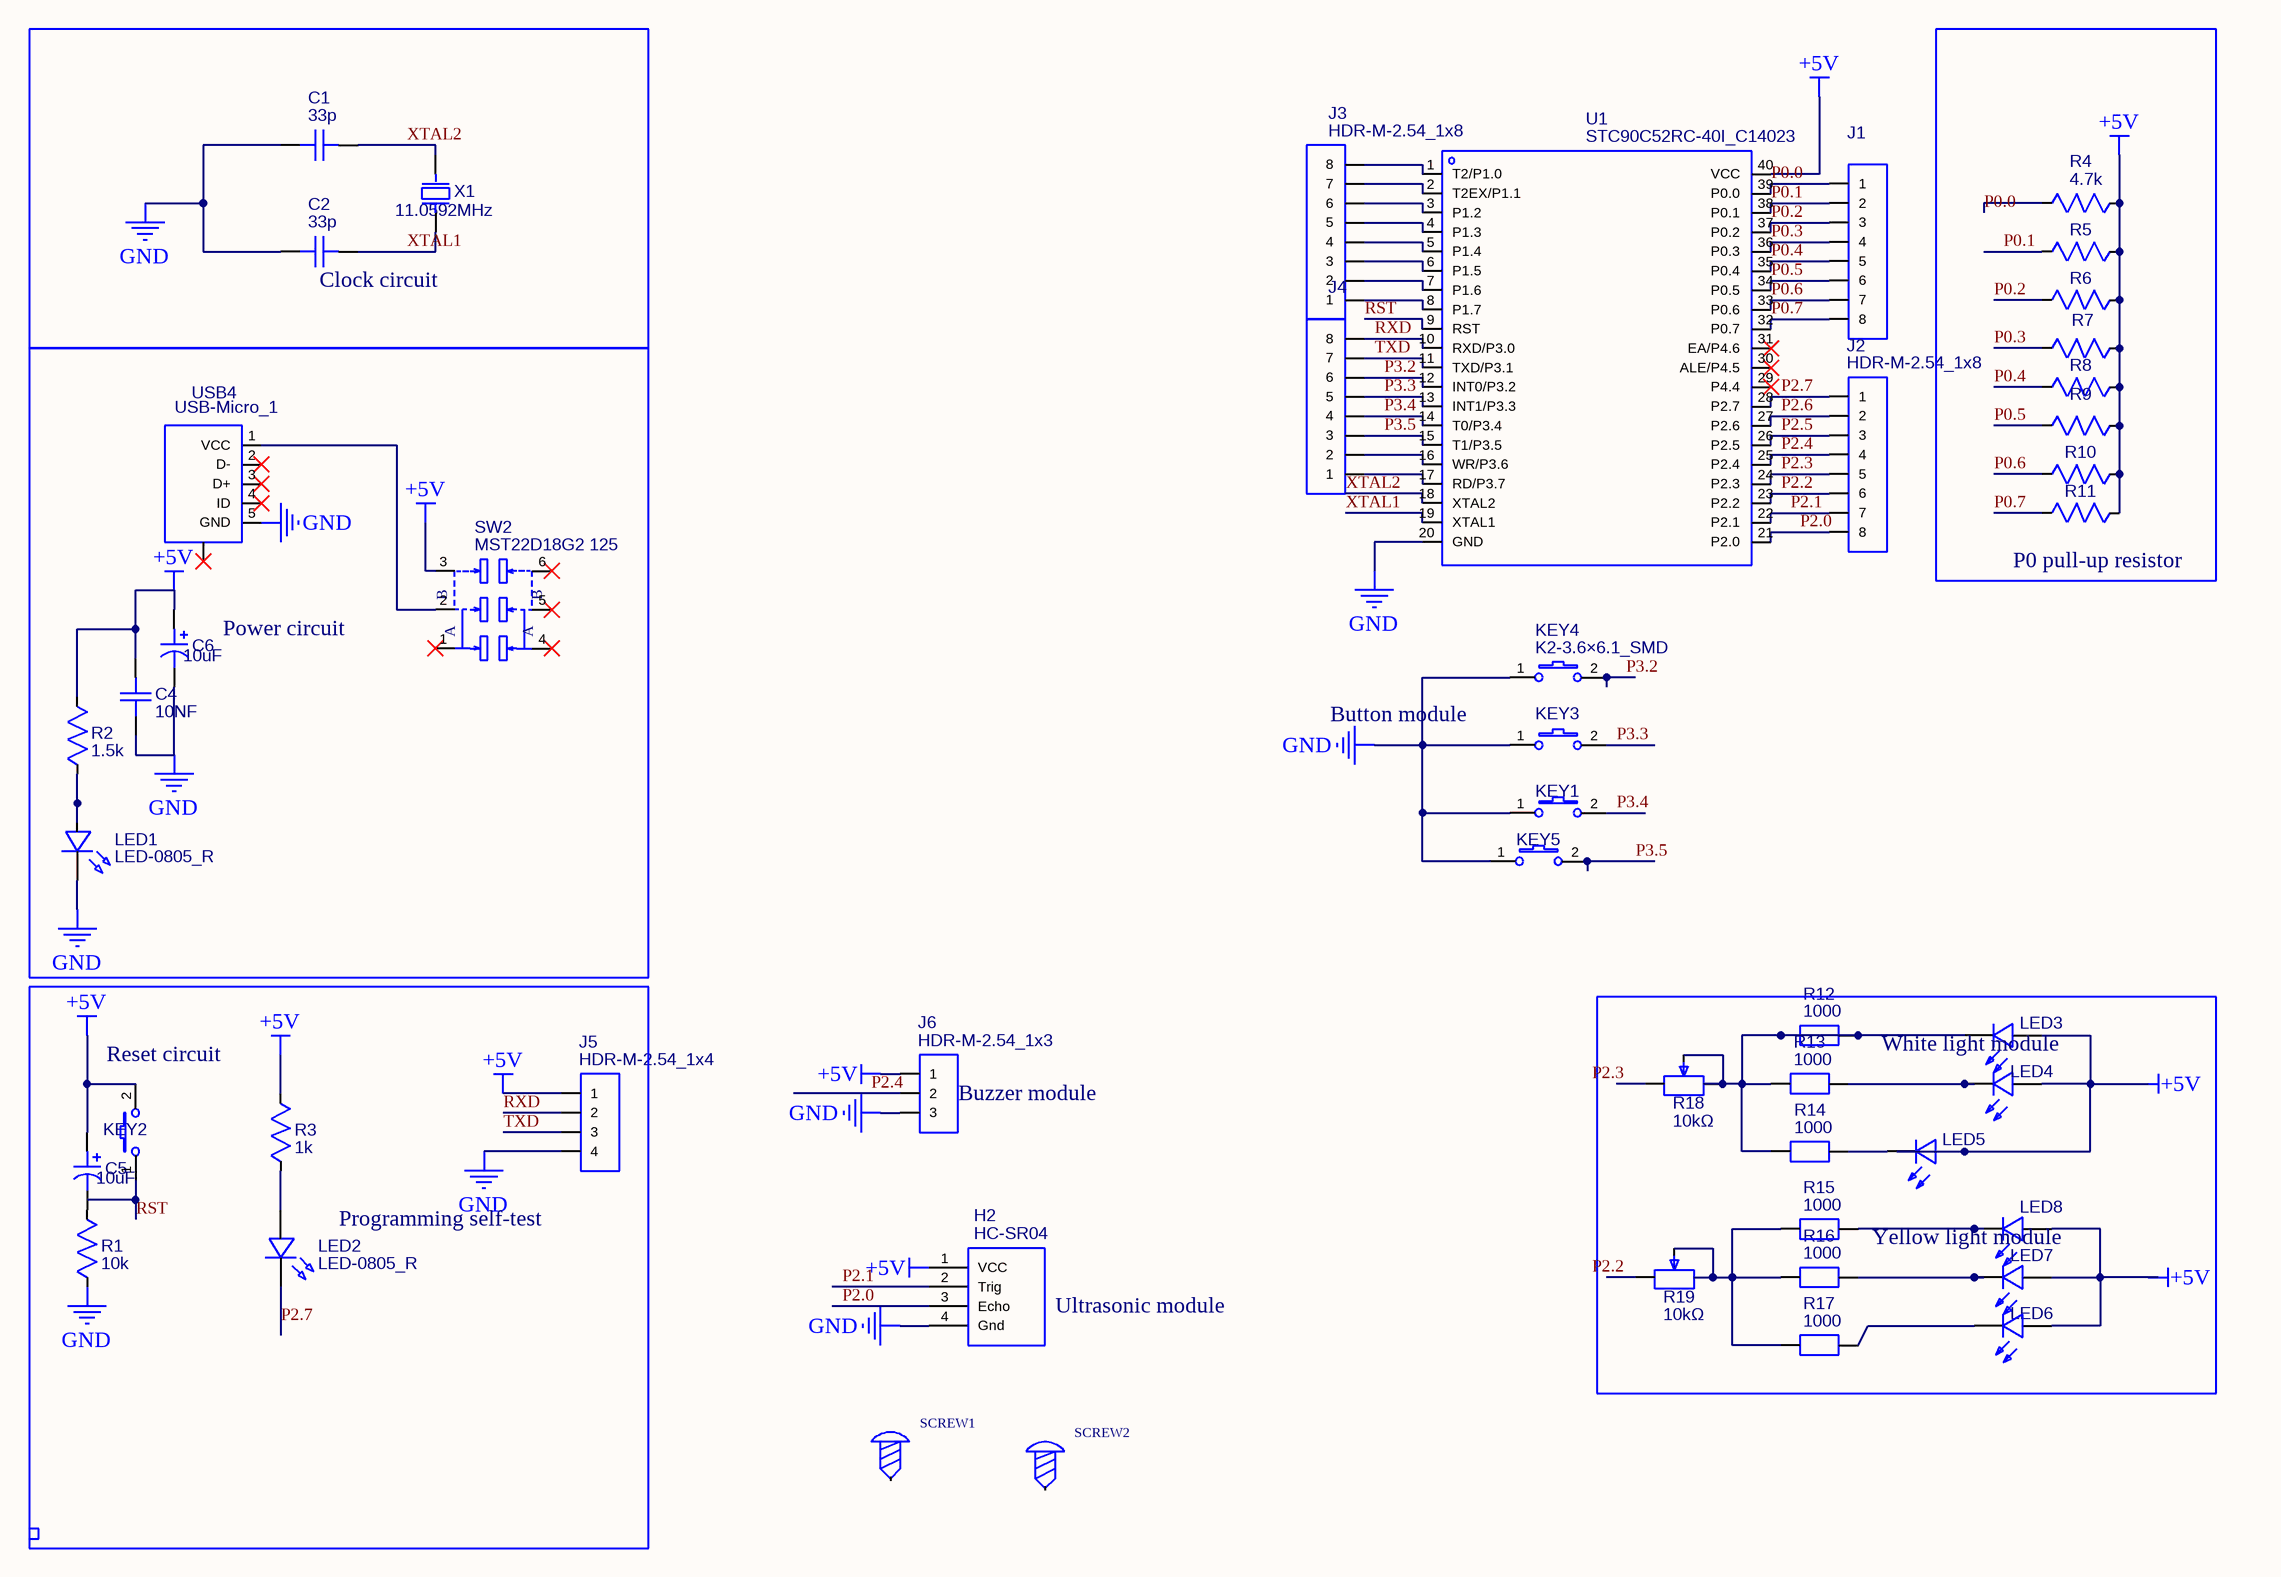
[diagram p0: MISC49914-3.schdoc]
# Altium project MISC49914-2.PrjPcb
1 sheet, 50 parts. Net scope: global (net labels, ports and power ports of the same name join across sheets).
Board file: MISC49914.pcbdoc

## Sheet MISC49914-3.schdoc
size 122 x 122 mm; Name: MISC49914; @Project Name: MISC49914; REV: 1.0; Date: 2023-03-04; Sheet: 1/1; Name: MISC49914; @Project Name: MISC49914; REV: 1.0; Date: 2023-03-04; Sheet: 1/1

### Parts
C1  33p  [C0805]
C2  33p  [C0805]
C4  10NF  [C0805]
C5  10uF  [CAP-TH_BD10.0-P5.00-D1.0-FD]
C6  10uF  [CAP-TH_BD10.0-P5.00-D1.0-FD]
H2  HC-SR04  [HC-SR04]
J1  HDR-M-2.54_1x8  [HDR-M-2.54_1X8]  (value not drawn)
J2  HDR-M-2.54_1x8  [HDR-M-2.54_1X8]
J3  HDR-M-2.54_1x8  [HDR-M-2.54_1X8]
J4  HDR-M-2.54_1x8  [HDR-M-2.54_1X8]  (value not drawn)
J5  HDR-M-2.54_1x4  [HDR-M-2.54_1X4]
J6  HDR-M-2.54_1x3  [HDR-M-2.54_1X3]
KEY1  K2-3.6×6.1_SMD  [KEY-SMD_2P-L6.2-W3.6-LS8.0]  (value not drawn)
KEY2  K2-3.6×6.1_SMD  [KEY-SMD_2P-L6.2-W3.6-LS8.0]  (value not drawn)
KEY3  K2-3.6×6.1_SMD  [KEY-SMD_2P-L6.2-W3.6-LS8.0]  (value not drawn)
KEY4  K2-3.6×6.1_SMD  [KEY-SMD_2P-L6.2-W3.6-LS8.0]
KEY5  K2-3.6×6.1_SMD  [KEY-SMD_2P-L6.2-W3.6-LS8.0]  (value not drawn)
LED1  LED-0805_R  [LED0805_RED]
LED2  LED-0805_R  [LED0805_RED]
LED3  204-10SDRD/S530-A3-L  [LED-TH_BD3.8-P2.54-FD]  (value not drawn)
LED4  204-10SDRD/S530-A3-L  [LED-TH_BD3.8-P2.54-FD]  (value not drawn)
LED5  204-10SDRD/S530-A3-L  [LED-TH_BD3.8-P2.54-FD]  (value not drawn)
LED6  204-10SDRD/S530-A3-L  [LED-TH_BD3.8-P2.54-FD]  (value not drawn)
LED7  204-10SDRD/S530-A3-L  [LED-TH_BD3.8-P2.54-FD]  (value not drawn)
LED8  204-10SDRD/S530-A3-L  [LED-TH_BD3.8-P2.54-FD]  (value not drawn)
R1  10k  [R0805]
R2  1.5k  [R0805]
R3  1k  [R0805]
R4  4.7k  [R0805]
R5  4.7k  [R0805]  (value not drawn)
R6  4.7k  [R0805]  (value not drawn)
R7  4.7k  [R0805]  (value not drawn)
R8  4.7k  [R0805]  (value not drawn)
R9  4.7k  [R0805]  (value not drawn)
R10  4.7k  [R0805]  (value not drawn)
R11  4.7k  [R0805]  (value not drawn)
R12  1000  [R0603]
R13  1000  [R0603]
R14  1000  [R0603]
R15  1000  [R0603]
R16  1000  [R0603]
R17  1000  [R0603]
R18  10kΩ  [RES-ADJ-TH_3296W]
R19  10kΩ  [RES-ADJ-TH_3296W]
SCREW1  (no value)  [M2螺丝]
SCREW2  (no value)  [M2螺丝]
SW2  MST22D18G2 125  [SW-SMD_MST22D18G2]
U1  STC90C52RC-40I_C14023  [DIP-40_L52.0-W13.7-P2.54-LS15.2-BL]
USB4  USB-Micro_1  [MICRO-USB-SMD_5P-P0.65-H-F_C10418]
X1  11.0592MHz  [OSC-TH_L10.0-W4.5-P5.00]

### Blocks framed on the sheet
Clock circuit: C1 C2 X1
P0 pull-up resistor: R4-R11
Power circuit: C4 C6 LED1 R2 SW2 USB4

### Nets
+5V: C4.2 C5.1 C6.1 H2.1(VCC) J5.1 J6.1 KEY2.2 LED3.1(A) LED4.1(A) LED5.1(A) LED6.1(A) LED7.1(A) LED8.1(A) R2.2 R3.2 R4.2 R5.2 R6.2 R7.2 R8.2 R9.2 R10.2 R11.2 SW2.3 U1.40(VCC)
GND: C1.1 C2.1 C4.1 C6.2 H2.4(Gnd) J5.4 J6.3 KEY1.1 KEY3.1 KEY4.1 KEY5.1 LED1.2 R1.1 U1.20(GND) USB4.5(GND)
P0.0: J1.1 R4.1 U1.39(P0.0)
P0.1: J1.2 R5.1 U1.38(P0.1)
P0.2: J1.3 R6.1 U1.37(P0.2)
P0.3: J1.4 R7.1 U1.36(P0.3)
P0.4: J1.5 R8.1 U1.35(P0.4)
P0.5: J1.6 R9.1 U1.34(P0.5)
P0.6: J1.7 R10.1 U1.33(P0.6)
P0.7: J1.8 R11.1 U1.32(P0.7)
P2.0: H2.3(Echo) J2.8 U1.21(P2.0)
P2.1: H2.2(Trig) J2.7 U1.22(P2.1)
P2.2: J2.6 R19.3 U1.23(P2.2)
P2.3: J2.5 R18.3 U1.24(P2.3)
P2.4: J2.4 J6.2 U1.25(P2.4)
P2.5: J2.3 U1.26(P2.5)
P2.6: J2.2 U1.27(P2.6)
P2.7: J2.1 LED2.2 U1.28(P2.7)
P3.2: J4.6 KEY4.2 U1.12(INT0/P3.2)
P3.3: J4.5 KEY3.2 U1.13(INT1/P3.3)
P3.4: J4.4 KEY1.2 U1.14(T0/P3.4)
P3.5: J4.3 KEY5.2 U1.15(T1/P3.5)
RST: KEY2.1 U1.9(RST)
RXD: J4.8 J5.2 U1.10(RXD/P3.0)
TXD: J4.7 J5.3 U1.11(TXD/P3.1)
XTAL1: C2.2 U1.19(XTAL1) X1.2(OSC2)
XTAL2: C1.2 U1.18(XTAL2) X1.1(OSC1)
NetC5_2: C5.2 R1.2
NetJ3_1: J3.1 U1.8(P1.7)
NetJ3_2: J3.2 U1.7(P1.6)
NetJ3_3: J3.3 U1.6(P1.5)
NetJ3_4: J3.4 U1.5(P1.4)
NetJ3_5: J3.5 U1.4(P1.3)
NetJ3_6: J3.6 U1.3(P1.2)
NetJ3_7: J3.7 U1.2(T2EX/P1.1)
NetJ3_8: J3.8 U1.1(T2/P1.0)
NetJ4_1: J4.1 U1.17(RD/P3.7)
NetJ4_2: J4.2 U1.16(WR/P3.6)
NetLED1_1: LED1.1 R2.1
NetLED2_1: LED2.1 R3.1
NetLED3_2: LED3.2(C) R13.1
NetLED4_2: LED4.2(C) R12.1 R12.2 R13.2 R14.2 R18.1 R18.2
NetLED5_2: LED5.2(C) R14.1
NetLED6_2: LED6.2(C) R15.1
NetLED7_2: LED7.2(C) R16.1
NetLED8_2: LED8.2(C) R17.1
NetR15_2: R15.2 R16.2 R17.2 R19.1 R19.2
NetSW2_2: SW2.2 USB4.1(VCC)

Not connected (* = marked no-connect by the designer): SCREW1 1; SCREW2 1; SW2 1* 4* 5* 6*; U1 29(P4.4)* 30(ALE/P4.5)* 31(EA/P4.6)*; USB4 0(MTN)* 2(D-)* 3(D+)* 4(ID)*

### Notes on the sheet
- Button module
- Reset circuit
- (near J6) Buzzer module
- (near LED4) White light module
- Programming self-test
- Ultrasonic module
- (near LED6) Yellow light module
- 1
- 2
- 3
- 4
- 5
- A
- B
- TITLE:
- Company:
- Sheet:
- REV:
- 1.0
- 1/1
- C
- Date:
- 2023-03-04
- Drawn By:
- D

### Library data of the parts
C1 = 33p: Convert to PCB: yes; UniqueId: ggeddfa5fd55caeadc4; Origin Footprint: C0805; Device: 33p; Symbol: 33p; Add into BOM: yes; FootprintName: C0805
C2 = 33p: Convert to PCB: yes; UniqueId: gge2aa6282be282581d; Origin Footprint: C0805; Device: 33p; Symbol: 33p; Add into BOM: yes; FootprintName: C0805
C4 = 10NF: Convert to PCB: yes; UniqueId: gge76a4c20b20eff667; Origin Footprint: C0805; Device: 10NF; Symbol: 10NF; Add into BOM: yes; FootprintName: C0805
C5 = EGS2GM100G12OTG: Manufacturer: AISHI(艾华集团); Convert to PCB: yes; UniqueId: gged4bc82e121489abd; Origin Footprint: CAP-TH_BD10.0-P5.00-D1.0-FD; Device: EGS2GM100G12OTG; Symbol: 10uF; Add into BOM: yes; Supplier: LCSC; SupplierPart: C724525; ManufacturerPart: EGS2GM100G12OTG; JLCPCB Part Class: Extended Part; FootprintName: CAP-TH_BD10.0-P5.00-D1.0-FD
C6 = EGS2GM100G12OTG: Manufacturer: AISHI(艾华集团); Convert to PCB: yes; UniqueId: gge2c11046f6bb86f1c; Origin Footprint: CAP-TH_BD10.0-P5.00-D1.0-FD; Device: EGS2GM100G12OTG; Symbol: 10uF; Add into BOM: yes; Supplier: LCSC; SupplierPart: C724525; ManufacturerPart: EGS2GM100G12OTG; JLCPCB Part Class: Extended Part; FootprintName: CAP-TH_BD10.0-P5.00-D1.0-FD
H2 = HC-SR04: Convert to PCB: yes; UniqueId: ggeceb1d04a11f585b4; Origin Footprint: HC-SR04; Device: HC-SR04; Symbol: HC-SR04; Add into BOM: yes; FootprintName: HC-SR04
J1 = HDR-M-2.54_1x8: Convert to PCB: yes; UniqueId: gge4f54badb484e97b8; Origin Footprint: HDR-M-2.54_1X8; Device: HDR-M-2.54_1x8; Symbol: HDR-M-2.54_1x8; Add into BOM: yes; SupplierPart: C190820; Supplier: LCSC; FootprintName: HDR-M-2.54_1X8
J2 = HDR-M-2.54_1x8: Convert to PCB: yes; UniqueId: gge20151e8849c19d5a; Origin Footprint: HDR-M-2.54_1X8; Device: HDR-M-2.54_1x8; Symbol: HDR-M-2.54_1x8; Add into BOM: yes; SupplierPart: C190820; Supplier: LCSC; FootprintName: HDR-M-2.54_1X8
J3 = HDR-M-2.54_1x8: Convert to PCB: yes; UniqueId: ggeffb33d07a586da4c; Origin Footprint: HDR-M-2.54_1X8; Device: HDR-M-2.54_1x8; Symbol: HDR-M-2.54_1x8; Add into BOM: yes; SupplierPart: C190820; Supplier: LCSC; FootprintName: HDR-M-2.54_1X8
J4 = HDR-M-2.54_1x8: Convert to PCB: yes; UniqueId: gge1950c038e9c0b450; Origin Footprint: HDR-M-2.54_1X8; Device: HDR-M-2.54_1x8; Symbol: HDR-M-2.54_1x8; Add into BOM: yes; SupplierPart: C190820; Supplier: LCSC; FootprintName: HDR-M-2.54_1X8
J5 = HDR-M-2.54_1x4: Convert to PCB: yes; UniqueId: gge7505e4ac977ca694; Origin Footprint: HDR-M-2.54_1X4; Device: HDR-M-2.54_1x4; Symbol: HDR-M-2.54_1x4; Add into BOM: yes; SupplierPart: C124378; Supplier: LCSC; FootprintName: HDR-M-2.54_1X4
J6 = HDR-M-2.54_1x3: Convert to PCB: yes; UniqueId: ggefe67ddca977efe93; Origin Footprint: HDR-M-2.54_1X3; Device: HDR-M-2.54_1x3; Symbol: HDR-M-2.54_1x3; Add into BOM: yes; SupplierPart: C180248; Supplier: LCSC; FootprintName: HDR-M-2.54_1X3
KEY1 = K2-1107ST-A4SW-06: 制造商: Hanyoung (Korea); Convert to PCB: yes; UniqueId: gge6ed31330496cf48b; Origin Footprint: KEY-SMD_2P-L6.2-W3.6-LS8.0; Device: K2-1107ST-A4SW-06; Symbol: K2-3.6×6.1_SMD; Add into BOM: yes; SupplierPart: C118141; Supplier: LCSC; ManufacturerPart: K2-1107ST-A4SW-06; FootprintName: KEY-SMD_2P-L6.2-W3.6-LS8.0
KEY2 = K2-1107ST-A4SW-06: 制造商: Hanyoung (Korea); Convert to PCB: yes; UniqueId: gge2a0448005aeded4f; Origin Footprint: KEY-SMD_2P-L6.2-W3.6-LS8.0; Device: K2-1107ST-A4SW-06; Symbol: K2-3.6×6.1_SMD; Add into BOM: yes; SupplierPart: C118141; Supplier: LCSC; ManufacturerPart: K2-1107ST-A4SW-06; FootprintName: KEY-SMD_2P-L6.2-W3.6-LS8.0
KEY3 = K2-1107ST-A4SW-06: 制造商: Hanyoung (Korea); Convert to PCB: yes; UniqueId: gge36d8e9403f70a06e; Origin Footprint: KEY-SMD_2P-L6.2-W3.6-LS8.0; Device: K2-1107ST-A4SW-06; Symbol: K2-3.6×6.1_SMD; Add into BOM: yes; SupplierPart: C118141; Supplier: LCSC; ManufacturerPart: K2-1107ST-A4SW-06; FootprintName: KEY-SMD_2P-L6.2-W3.6-LS8.0
KEY4 = K2-1107ST-A4SW-06: 制造商: Hanyoung (Korea); Convert to PCB: yes; UniqueId: gged006399c1d47c4d0; Origin Footprint: KEY-SMD_2P-L6.2-W3.6-LS8.0; Device: K2-1107ST-A4SW-06; Symbol: K2-3.6×6.1_SMD; Add into BOM: yes; SupplierPart: C118141; Supplier: LCSC; ManufacturerPart: K2-1107ST-A4SW-06; FootprintName: KEY-SMD_2P-L6.2-W3.6-LS8.0
KEY5 = K2-1107ST-A4SW-06: 制造商: Hanyoung (Korea); Convert to PCB: yes; UniqueId: gge5452d93a29099d09; Origin Footprint: KEY-SMD_2P-L6.2-W3.6-LS8.0; Device: K2-1107ST-A4SW-06; Symbol: K2-3.6×6.1_SMD; Add into BOM: yes; SupplierPart: C118141; Supplier: LCSC; ManufacturerPart: K2-1107ST-A4SW-06; FootprintName: KEY-SMD_2P-L6.2-W3.6-LS8.0
LED1 = 17-21SURC/S530-A3/TR8: Manufacturer: EVERLIGHT(台湾亿光); Convert to PCB: yes; UniqueId: gge6e977688b4c4456b; Origin Footprint: LED0805_RED; Device: 17-21SURC/S530-A3/TR8; Symbol: LED-0805_R; Add into BOM: yes; ManufacturerPart: 17-21SURC/S530-A3/TR8; SupplierPart: C72037; FootprintName: LED0805_RED
LED2 = 17-21SURC/S530-A3/TR8: Manufacturer: EVERLIGHT(台湾亿光); Convert to PCB: yes; UniqueId: gge2806d153729380c4; Origin Footprint: LED0805_RED; Device: 17-21SURC/S530-A3/TR8; Symbol: LED-0805_R; Add into BOM: yes; ManufacturerPart: 17-21SURC/S530-A3/TR8; SupplierPart: C72037; FootprintName: LED0805_RED
LED3 = 204-10SDRD/S530-A3-L: Manufacturer: EVERLIGHT(亿光); Convert to PCB: yes; UniqueId: gge1c4812dc0b201fda; Origin Footprint: LED-TH_BD3.8-P2.54-FD; Device: 204-10SDRD/S530-A3-L; Symbol: 204-10SDRD/S530-A3-L; Add into BOM: yes; Supplier: LCSC; ManufacturerPart: 204-10SDRD/S530-A3-L; SupplierPart: C84774; JLCPCB Part Class: Extended Part; FootprintName: LED-TH_BD3.8-P2.54-FD
LED4 = 204-10SDRD/S530-A3-L: Manufacturer: EVERLIGHT(亿光); Convert to PCB: yes; UniqueId: gge47435d56cf3ad1dc; Origin Footprint: LED-TH_BD3.8-P2.54-FD; Device: 204-10SDRD/S530-A3-L; Symbol: 204-10SDRD/S530-A3-L; Add into BOM: yes; Supplier: LCSC; ManufacturerPart: 204-10SDRD/S530-A3-L; SupplierPart: C84774; JLCPCB Part Class: Extended Part; FootprintName: LED-TH_BD3.8-P2.54-FD
LED5 = 204-10SDRD/S530-A3-L: Manufacturer: EVERLIGHT(亿光); Convert to PCB: yes; UniqueId: gge89f50a57f8133979; Origin Footprint: LED-TH_BD3.8-P2.54-FD; Device: 204-10SDRD/S530-A3-L; Symbol: 204-10SDRD/S530-A3-L; Add into BOM: yes; Supplier: LCSC; ManufacturerPart: 204-10SDRD/S530-A3-L; SupplierPart: C84774; JLCPCB Part Class: Extended Part; FootprintName: LED-TH_BD3.8-P2.54-FD
LED6 = 204-10SDRD/S530-A3-L: Manufacturer: EVERLIGHT(亿光); Convert to PCB: yes; UniqueId: gge513db9466068992b; Origin Footprint: LED-TH_BD3.8-P2.54-FD; Device: 204-10SDRD/S530-A3-L; Symbol: 204-10SDRD/S530-A3-L; Add into BOM: yes; Supplier: LCSC; ManufacturerPart: 204-10SDRD/S530-A3-L; SupplierPart: C84774; JLCPCB Part Class: Extended Part; FootprintName: LED-TH_BD3.8-P2.54-FD
LED7 = 204-10SDRD/S530-A3-L: Manufacturer: EVERLIGHT(亿光); Convert to PCB: yes; UniqueId: gge5aecfdf7b982d54e; Origin Footprint: LED-TH_BD3.8-P2.54-FD; Device: 204-10SDRD/S530-A3-L; Symbol: 204-10SDRD/S530-A3-L; Add into BOM: yes; Supplier: LCSC; ManufacturerPart: 204-10SDRD/S530-A3-L; SupplierPart: C84774; JLCPCB Part Class: Extended Part; FootprintName: LED-TH_BD3.8-P2.54-FD
LED8 = 204-10SDRD/S530-A3-L: Manufacturer: EVERLIGHT(亿光); Convert to PCB: yes; UniqueId: gge6723be1ad144d563; Origin Footprint: LED-TH_BD3.8-P2.54-FD; Device: 204-10SDRD/S530-A3-L; Symbol: 204-10SDRD/S530-A3-L; Add into BOM: yes; Supplier: LCSC; ManufacturerPart: 204-10SDRD/S530-A3-L; SupplierPart: C84774; JLCPCB Part Class: Extended Part; FootprintName: LED-TH_BD3.8-P2.54-FD
R1 = 10k: Convert to PCB: yes; UniqueId: gge2b7846e56ea7b434; Origin Footprint: R0805; Device: 10k; Symbol: 10k; Add into BOM: yes; FootprintName: R0805
R2 = 1.5k: Convert to PCB: yes; UniqueId: gge3ae89372b32b9042; Origin Footprint: R0805; Device: 1.5k; Symbol: 1.5k; Add into BOM: yes; FootprintName: R0805
R3 = 1k: Convert to PCB: yes; UniqueId: ggee0d0399772d173d2; Origin Footprint: R0805; Device: 1k; Symbol: 1k; Add into BOM: yes; FootprintName: R0805
R4 = 4.7k: Convert to PCB: yes; UniqueId: gge566a17a88b489960; Origin Footprint: R0805; Device: 4.7k; Symbol: 4.7k; Add into BOM: yes; FootprintName: R0805
R5 = 4.7k: Convert to PCB: yes; UniqueId: gge8e60508b856c24e5; Origin Footprint: R0805; Device: 4.7k; Symbol: 4.7k; Add into BOM: yes; FootprintName: R0805
R6 = 4.7k: Convert to PCB: yes; UniqueId: gge42c99a7c33e1aa67; Origin Footprint: R0805; Device: 4.7k; Symbol: 4.7k; Add into BOM: yes; FootprintName: R0805
R7 = 4.7k: Convert to PCB: yes; UniqueId: ggec85e47c78710c2dc; Origin Footprint: R0805; Device: 4.7k; Symbol: 4.7k; Add into BOM: yes; FootprintName: R0805
R8 = 4.7k: Convert to PCB: yes; UniqueId: gge35461d2c10540f0e; Origin Footprint: R0805; Device: 4.7k; Symbol: 4.7k; Add into BOM: yes; FootprintName: R0805
R9 = 4.7k: Convert to PCB: yes; UniqueId: gge2d233aec4856bc39; Origin Footprint: R0805; Device: 4.7k; Symbol: 4.7k; Add into BOM: yes; FootprintName: R0805
R10 = 4.7k: Convert to PCB: yes; UniqueId: ggee29d2a3e025a0491; Origin Footprint: R0805; Device: 4.7k; Symbol: 4.7k; Add into BOM: yes; FootprintName: R0805
R11 = 4.7k: Convert to PCB: yes; UniqueId: gge5f0982b0c73645ed; Origin Footprint: R0805; Device: 4.7k; Symbol: 4.7k; Add into BOM: yes; FootprintName: R0805
R12 = 1000: Convert to PCB: yes; UniqueId: ggeeb5e6458d58bf9ef; Origin Footprint: R0603; Device: 1000; Symbol: 1000; Add into BOM: yes; FootprintName: R0603
R13 = 1000: Convert to PCB: yes; UniqueId: ggef8e73dd396a52c87; Origin Footprint: R0603; Device: 1000; Symbol: 1000; Add into BOM: yes; FootprintName: R0603
R14 = 1000: Convert to PCB: yes; UniqueId: gge021b2f505cd858c1; Origin Footprint: R0603; Device: 1000; Symbol: 1000; Add into BOM: yes; FootprintName: R0603
R15 = 1000: Convert to PCB: yes; UniqueId: ggea4b3efd371e5a5b4; Origin Footprint: R0603; Device: 1000; Symbol: 1000; Add into BOM: yes; FootprintName: R0603
R16 = 1000: Convert to PCB: yes; UniqueId: ggeaa53703de138b791; Origin Footprint: R0603; Device: 1000; Symbol: 1000; Add into BOM: yes; FootprintName: R0603
R17 = 1000: Convert to PCB: yes; UniqueId: ggea5e033e2dd905ce1; Origin Footprint: R0603; Device: 1000; Symbol: 1000; Add into BOM: yes; FootprintName: R0603
R18 = 3296W-1-103LF: Manufacturer: BOURNS; Convert to PCB: yes; UniqueId: gge1264741f20652521; Resistance: 10K; Origin Footprint: RES-ADJ-TH_3296W; Device: 3296W-1-103LF; Symbol: 10kΩ; Add into BOM: yes; Supplier: LCSC; ManufacturerPart: 3296W-1-103LF; SupplierPart: C34846; JLCPCB Part Class: Extended Part; FootprintName: RES-ADJ-TH_3296W
R19 = 3296W-1-103LF: Manufacturer: BOURNS; Convert to PCB: yes; UniqueId: gge4f7fac8f7729baab; Resistance: 10K; Origin Footprint: RES-ADJ-TH_3296W; Device: 3296W-1-103LF; Symbol: 10kΩ; Add into BOM: yes; Supplier: LCSC; ManufacturerPart: 3296W-1-103LF; SupplierPart: C34846; JLCPCB Part Class: Extended Part; FootprintName: RES-ADJ-TH_3296W
SCREW1 SCREW2 = M2螺丝: Symbol: Screw hole; Device: M2 screw; ConvertToPcb: yes; AddInBom: yes; Supplier Footprint: 插件; FootprintName: M2 screw
SW2 = MST22D18G2 125: Manufacturer: SHOU HAN(首韩); Convert to PCB: yes; UniqueId: ggef315a8375b69cc31; Origin Footprint: SW-SMD_MST22D18G2; Device: MST22D18G2 125; Symbol: MST22D18G2 125; Add into BOM: yes; Supplier: LCSC; SupplierPart: C2906280; ManufacturerPart: MST22D18G2 125; JLCPCB Part Class: Extended Part; FootprintName: SW-SMD_MST22D18G2
U1 = STC90C52RC-40I: Manufacturer: STC; Convert to PCB: yes; UniqueId: gge33d461692f6a39ed; Origin Footprint: DIP-40_L52.0-W13.7-P2.54-LS15.2-BL; Device: STC90C52RC-40I; Symbol: STC90C52RC-40I_C14023; Add into BOM: yes; Supplier: LCSC; ManufacturerPart: STC90C52RC-40I; SupplierPart: C14023; FootprintName: DIP-40_L52.0-W13.7-P2.54-LS15.2-BL
USB4 = USB-Micro_1: Manufacturer: ValuePro; Convert to PCB: yes; UniqueId: gge0185afe60705ab00; Origin Footprint: MICRO-USB-SMD_5P-P0.65-H-F_C10418; Device: USB-Micro_1; Symbol: USB-Micro_1; Add into BOM: yes; SupplierPart: C10418; Supplier: LCSC; FootprintName: MICRO-USB-SMD_5P-P0.65-H-F_C10418
X1 = X49UD110592MSD2SC: Manufacturer: YXC; Convert to PCB: yes; UniqueId: gge9fc9b0276ec47414; Origin Footprint: OSC-TH_L10.0-W4.5-P5.00; Device: X49UD110592MSD2SC; Symbol: 11.0592MHz; Add into BOM: yes; Supplier: LCSC; ManufacturerPart: X49UD110592MSD2SC; SupplierPart: C2194; FootprintName: OSC-TH_L10.0-W4.5-P5.00